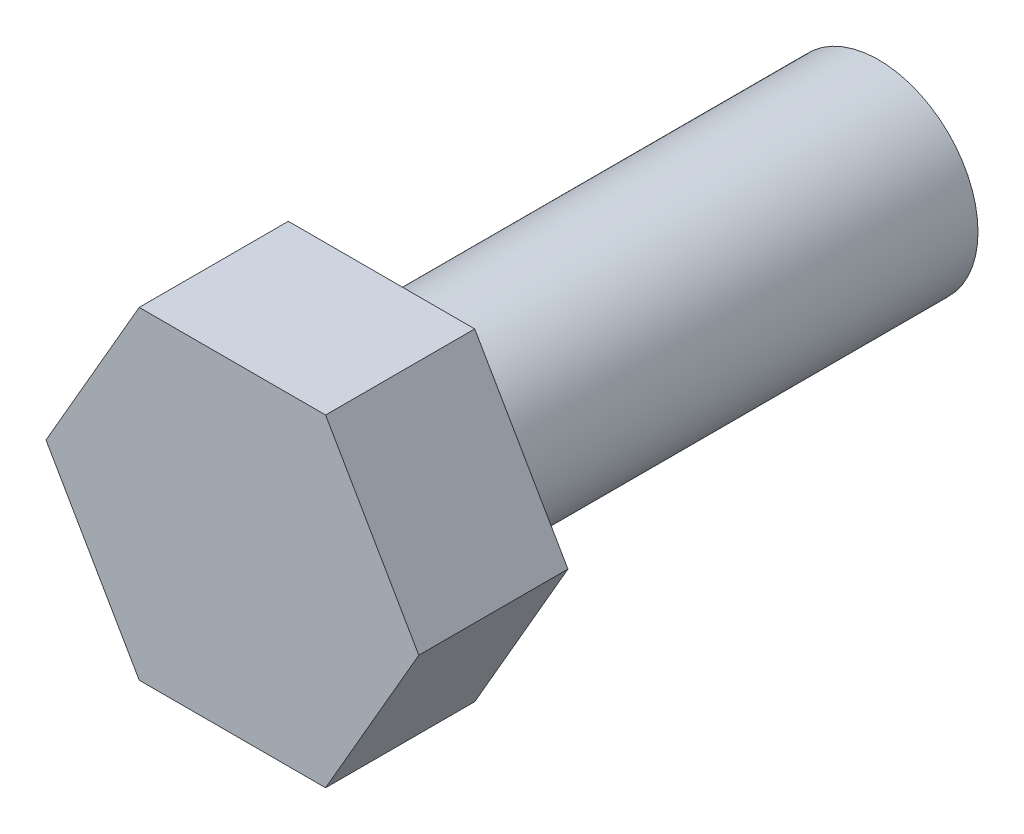
from build123d import *

# Parameters (mm, degrees)
SKETCH1_R           = 4
BOSS_EXTRUDE1_DEPTH = 20
BOSS_EXTRUDE2_DEPTH = 6


with BuildPart() as part:
    # Sketch1 → Boss-Extrude1 (new body)
    with BuildSketch(Plane.XY):
        Circle(SKETCH1_R)
    extrude(amount=BOSS_EXTRUDE1_DEPTH)

    # Sketch2 → Boss-Extrude2 (add)
    with BuildSketch(Plane.XY.offset(20)):
        Polygon((-3.75, 6.495190528), (-7.5, 0), (-3.75, -6.495190528), (3.75, -6.495190528), (7.5, 0), (3.75, 6.495190528), align=None)
    extrude(amount=BOSS_EXTRUDE2_DEPTH)


solid = part.part
